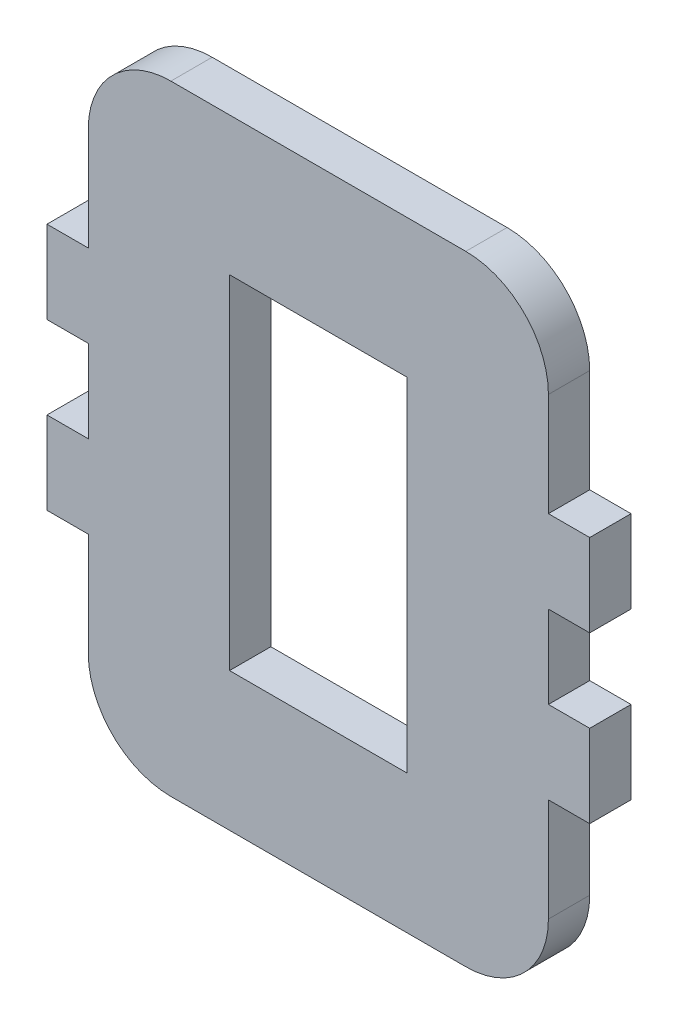
SolidWorks part; units mm, degrees
ref_plane "前视基准面" through (0, 0, 0) normal (0, 0, 1) x (1, 0, 0)
ref_plane "上视基准面" through (0, 0, 0) normal (0, 1, 0) x (1, 0, 0)
ref_plane "右视基准面" through (0, 0, 0) normal (1, 0, 0) x (0, 0, -1)
sketch "草图1" plane through (0, 0, 0) normal (0, 0, 1) x (1, 0, 0)
  line L0 (-27.85, 15) -> (-27.85, 37.5)
  line L1 (0, 1000) -> (0, 37.5) construction
  line L2 (27.85, -37.5) -> (27.85, -15)
  line L3 (-27.85, -37.5) -> (27.85, -37.5)
  line L4 (-32.85, -15) -> (-32.85, -5)
  line L5 (-27.85, 37.5) -> (27.85, 37.5)
  line L6 (32.85, -15) -> (32.85, -5)
  line L9 (32.85, -15) -> (27.85, -15)
  line L10 (32.85, -15) -> (32.85, -5)
  line L11 (32.85, -5) -> (27.85, -5)
  line L13 (32.85, 5) -> (27.85, 5)
  line L14 (32.85, 5) -> (32.85, 15)
  line L15 (32.85, 15) -> (27.85, 15)
  line L17 (-32.85, -5) -> (-27.85, -5)
  line L19 (-32.85, -15) -> (-27.85, -15)
  line L20 (-32.85, -15) -> (-32.85, -5)
  line L21 (-32.85, 15) -> (-27.85, 15)
  line L23 (-32.85, 5) -> (-27.85, 5)
  line L24 (-32.85, 5) -> (-32.85, 15)
  line L25 (-27.85, -37.5) -> (-27.85, -15)
  line L26 (32.85, 5) -> (32.85, 15)
  line L27 (-32.85, 5) -> (-32.85, 15)
  line L29 (-27.85, -5) -> (-27.85, 5)
  line L30 (27.85, 15) -> (27.85, 38.0633)
  line L31 (27.85, -5) -> (27.85, 5)
  line L32 (0, -37.5) -> (0, -1072.4038) construction
  point P1 (0, 0)
  dimension "D3" = 10
  dimension "D4" = 10
  dimension "D5" = 5
extrude "凸台-拉伸1" add sketch "草图1" along normal blind 5 contours L11 L31 L13 L14 L15 L30 L5 L0 L21 L24 L23 L29 L17 L4 L19 L25 L3 L2 L9 L6
sketch "草图2" plane through (0, 0, 5) normal (0, 0, 1) x (1, 0, 0)
  line L0 (0, 20.75) -> (0, -20.75) construction
  line L1 (10.75, 0) -> (-10.75, 0) construction
  line L3 (-10.75, -20.75) -> (10.75, -20.75)
  line L4 (-10.75, -20.75) -> (-10.75, 20.75)
  line L5 (-10.75, 20.75) -> (10.75, 20.75)
  line L6 (10.75, -20.75) -> (10.75, 20.75)
  line L7 (-10.75, -20.75) -> (10.75, 20.75) construction
  line L8 (-10.75, 20.75) -> (10.75, -20.75) construction
  point P10 (0, 0)
  dimension "D2" = 41.5
  dimension "D3" = 21.5
extrude "切除-拉伸1" cut sketch "草图2" against normal blind 5
fillet "圆角1" radius 10 4 edges at (27.85, -37.5, 2.5) (-27.85, -37.5, 2.5) (-27.85, 37.5, 2.5) (27.85, 37.5, 2.5)
